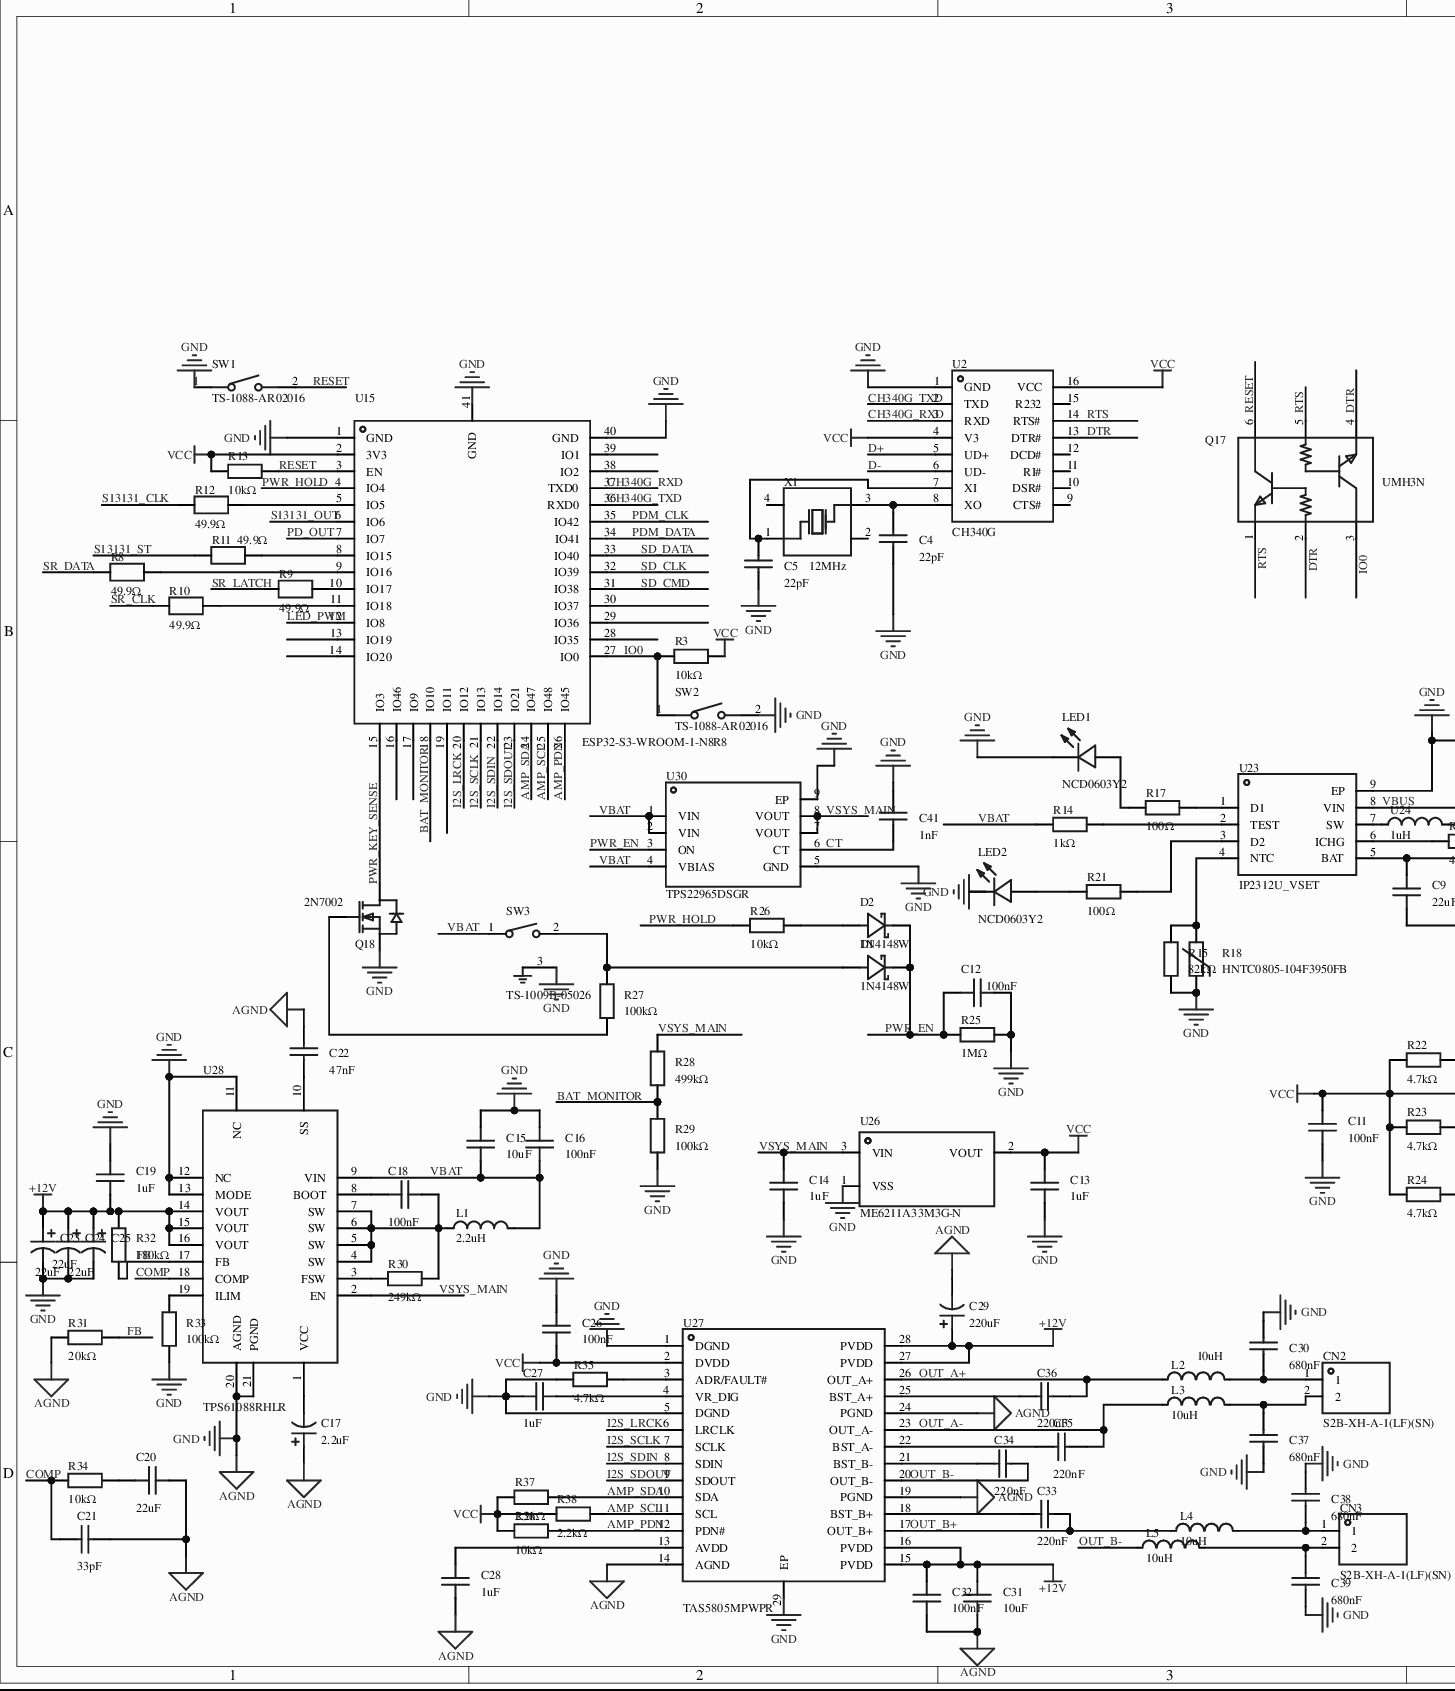
[diagram p0: MISC75432-3.schdoc, left]
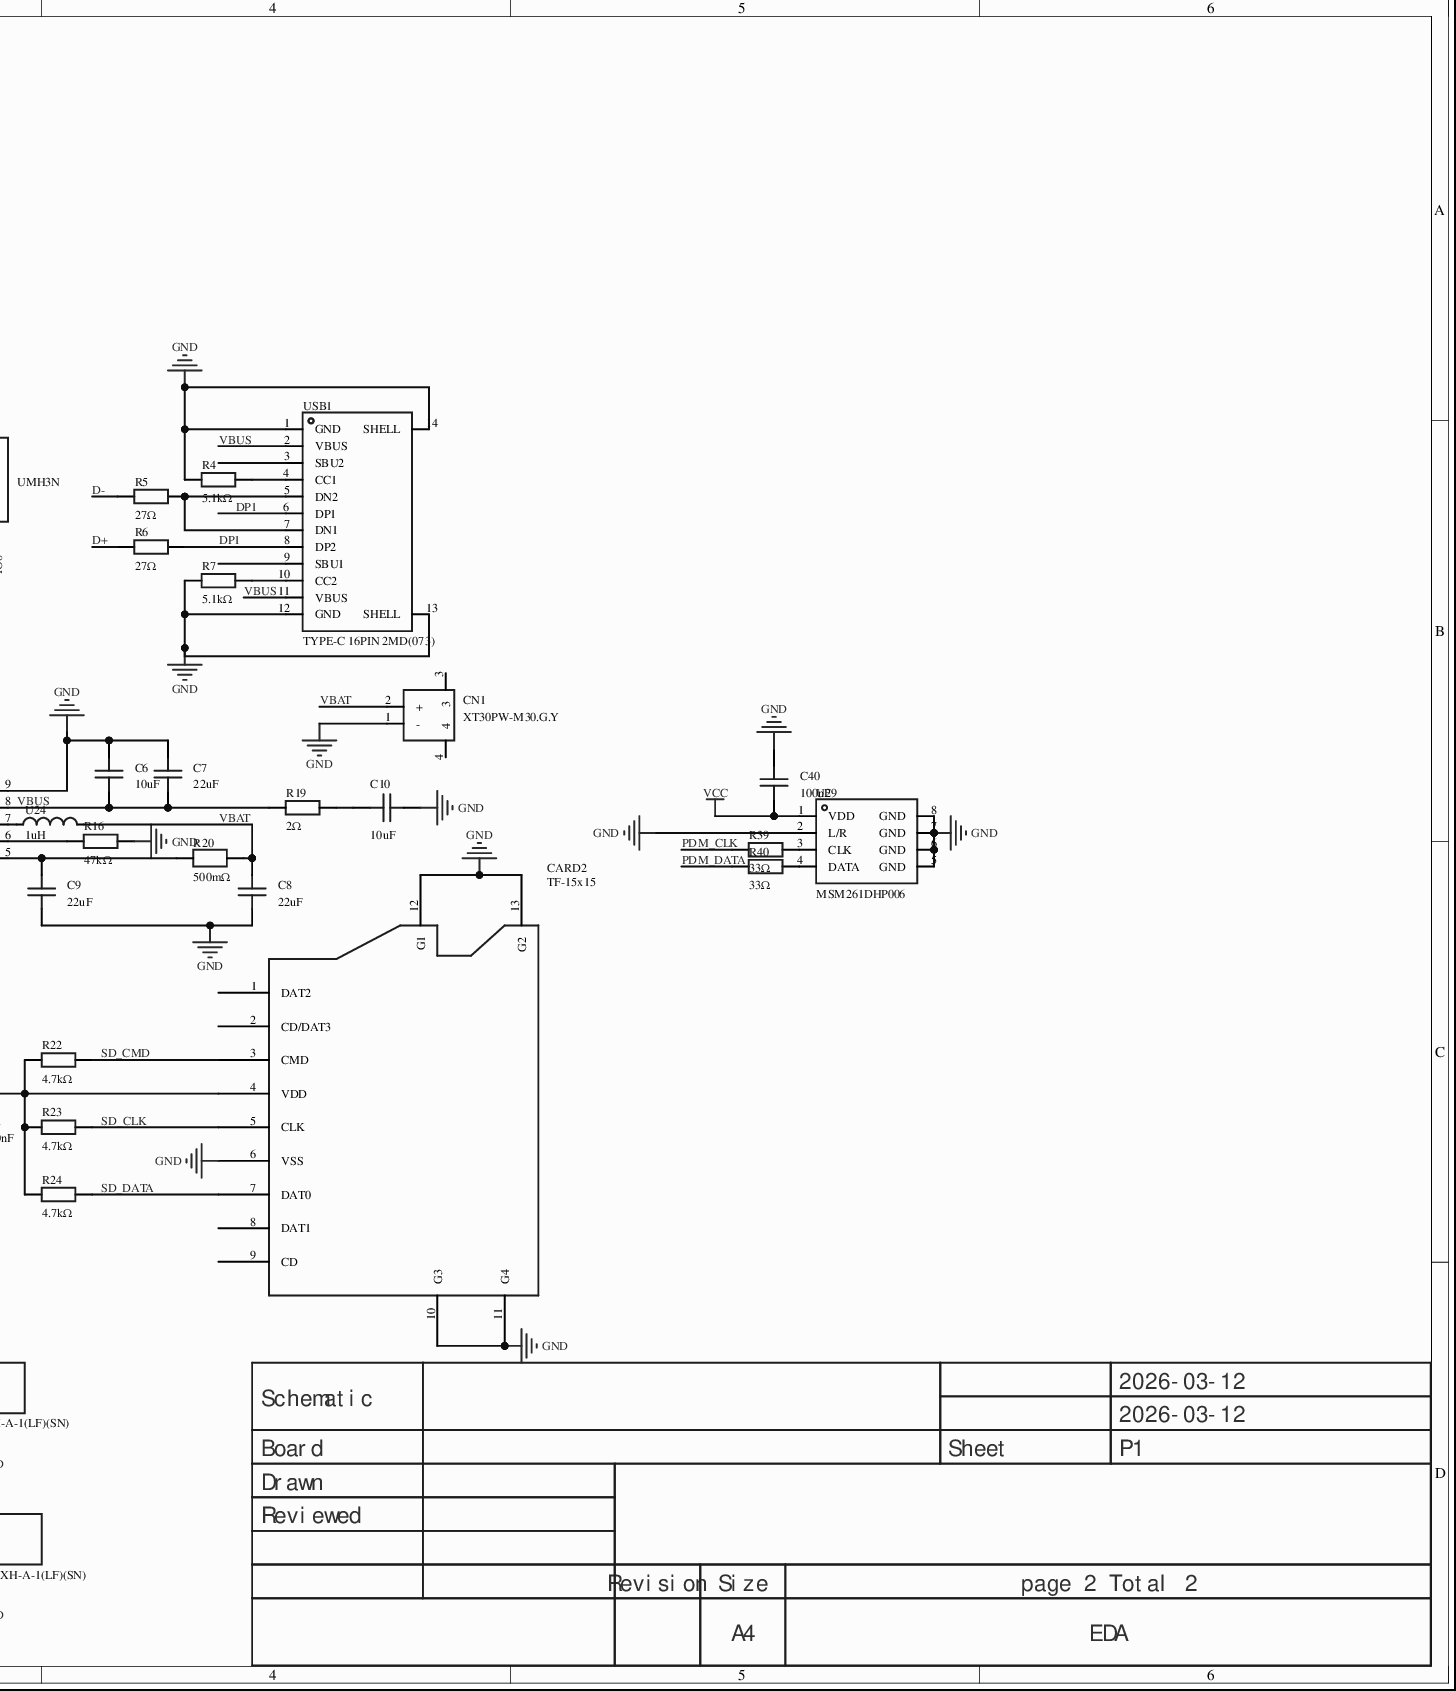
[diagram p1: MISC75432-3.schdoc, right]
# Altium project MISC75432-2.PrjPcb (part 1 of 3)
2 sheets, 150 parts. Net scope: global (net labels, ports and power ports of the same name join across sheets).
Board file: MISC75432.pcbdoc
Sheets:
  MISC75432-3.schdoc
  MISC75432-4.schdoc

## Sheet MISC75432-3.schdoc
size 424 x 254 mm; Version: V1.0; @Project Name: MISC75432; @Update Date: 2026-03-12; @Create Date: 2026-03-12; @Board Name: MISC75432; @Create Time: 13:14:40; @Page Count: 2; @Page No: 2; @Schematic Name: MISC75432; @Update Time: 13:14:40; Size: A4

### Parts
C4  22pF  [C0603]
C5  22pF  [C0603]
C6  10uF  [C0603]
C7  22uF  [C0603]
C8  22uF  [C0603]
C9  22uF  [C0603]
C10  10uF  [C0603]
C11  100nF  [C0603]
C12  100nF  [C0603]
C13  1uF  [C0603]
C14  1uF  [C0603]
C15  10uF  [C0603]
C16  100nF  [C0603]
C17  2.2uF  [CAP-SMD_BD5.0-L5.3-W5.3-LS6.0-FD]
C18  100nF  [C0603]
C19  1uF  [C0603]
C20  22uF  [C0603]
C21  33pF  [C0603]
C22  47nF  [C0603]
C23  22uF  [CAP-SMD_BD5.0-L5.3-W5.3-LS6.3-FD-1]
C24  22uF  [CAP-SMD_BD5.0-L5.3-W5.3-LS6.3-FD-1]
C25  22uF  [CAP-SMD_BD5.0-L5.3-W5.3-LS6.3-FD-1]
C26  100nF  [C0603]
C27  1uF  [C0603]
C28  1uF  [C0603]
C29  220uF  [CAP-SMD_BD6.3-L6.6-W6.6-LS7.3-FD-H7.7]
C30  680nF  [C0603]
C31  10uF  [C0603]
C32  100nF  [C0603]
C33  220nF  [C0603]
C34  220nF  [C0603]
C35  220nF  [C0603]
C36  220nF  [C0603]
C37  680nF  [C0603]
C38  680nF  [C0603]
C39  680nF  [C0603]
C40  100nF  [C0603]
C41  1nF  [C0603]
CARD2  TF-15x15  [TF-SMD_TF-15-15]
CN1  XT30PW-M30.G.Y  [CONN-TH_XT30PW-M]
CN2  S2B-XH-A-1(LF)(SN)  [CONN-TH_S2B-XH-A-1-LF-SN]
CN3  S2B-XH-A-1(LF)(SN)  [CONN-TH_S2B-XH-A-1-LF-SN]
D1  1N4148W  [SOD-123_L2.7-W1.6-LS3.7-FD]
D2  1N4148W  [SOD-123_L2.7-W1.6-LS3.7-FD]
L1  2.2uH  [IND-SMD_L4.6-W4.1_MHCI04015]
L2  10uH  [IND-SMD_L7.3-W6.8]
L3  10uH  [IND-SMD_L7.3-W6.8]
L4  10uH  [IND-SMD_L7.3-W6.8]
L5  10uH  [IND-SMD_L7.3-W6.8]
LED1  NCD0603Y2  [LED0603-RD]
LED2  NCD0603Y2  [LED0603-RD]
Q17  UMH3N  [SC-70-6_L2.2-W1.3-P0.65-LS2.1-BR]
Q18  2N7002  [SOT-23-3_L2.9-W1.3-P1.90-LS2.4-BR]
R3  10kΩ  [R0603]
R4  5.1kΩ  [R0603]
R5  27Ω  [R0603]
R6  27Ω  [R0603]
R7  5.1kΩ  [R0603]
R8  49.9Ω  [R0603]
R9  49.9Ω  [R0603]
R10  49.9Ω  [R0603]
R11  49.9Ω  [R0603]
R12  49.9Ω  [R0603]
R13  10kΩ  [R0603]
R14  1kΩ  [R0603]
R15  82kΩ  [R0603]
R16  47kΩ  [R0603]
R17  100Ω  [R0603]
R18  HNTC0805-104F3950FB  [R0805]
R19  2Ω  [R0603]
R20  500mΩ  [R1206]
R21  100Ω  [R0603]
R22  4.7kΩ  [R0603]
R23  4.7kΩ  [R0603]
R24  4.7kΩ  [R0603]
R25  1MΩ  [R0603]
R26  10kΩ  [R0603]
R27  100kΩ  [R0603]
R28  499kΩ  [R0603]
R29  100kΩ  [R0603]
R30  249kΩ  [R0603]
R31  20kΩ  [R0603]
R32  180kΩ  [R0603]
R33  100kΩ  [R0603]
R34  10kΩ  [R0603]
R35  4.7kΩ  [R0603]
R36  10kΩ  [R0603]
R37  2.2kΩ  [R0603]
R38  2.2kΩ  [R0603]
R39  33Ω  [R0603]
R40  33Ω  [R0603]
SW1  TS-1088-AR02016  [SW-SMD_L3.9-W3.0-P4.45]
SW2  TS-1088-AR02016  [SW-SMD_L3.9-W3.0-P4.45]
SW3  TS-1009B-05026  [SW-TH_3P-L4.5-W3.8-P3.10-LS1.9_TS-1009B-05026]
U2  CH340G  [SOIC-16_L9.9-W3.9-P1.27-LS6.0-BL]
U15  ESP32-S3-WROOM-1-N8R8  [WIRELM-SMD_ESP32-S3-WROOM-1]
U23  IP2312U_VSET  [SOP-8_L4.9-W3.9-P1.27-LS6.0-BL-EP]
U24  1uH  [IND-SMD_L2.5-W2.0-VLS252012CX-150M]
U26  ME6211A33M3G-N  [SOT-23-3_L2.9-W1.6-P1.90-LS2.8-BR]
U27  TAS5805MPWPR  [HTSSOP-28_L9.7-W4.4-P0.65-LS6.4-BL-EP]
U28  TPS61088RHLR  [VQFN-20_L4.6-W3.6-P0.50-BL]
U29  MSM261DHP006  [QFN-8_L4.0-W3.0_WMM7040DTHN0-8-TR]
U30  TPS22965DSGR  [UDFN-8_L2.0-W2.0-P0.50-TL-EP]
USB1  TYPE-C 16PIN 2MD(073)  [USB-C-SMD_TYPE-C-6PIN-2MD-073]
X1  12MHz  [CRYSTAL-SMD_4P-L3.2-W2.5-BL]

### Nets
+12V: C19.1 C23.1 C24.1 C25.1 C29.1 C31.2 C32.2 R32.2 U27.15(PVDD) U27.16(PVDD) U27.27(PVDD) U27.28(PVDD) U28.14(VOUT) U28.15(VOUT) U28.16(VOUT)
GND: C4.1 C5.1 C6.2 C7.2 C8.1 C9.1 C10.2 C11.1 C12.2 C13.1 C14.1 C15.2 C16.2 C17.1 C19.2 C20.2 C21.2 C22.2 C23.2 C24.2 C25.2 C26.2 C27.2 C28.1 C29.2 C30.2 C31.1 C32.1 C37.1 C38.2 C39.1 C40.2 C41.2 CARD2.6(VSS) CARD2.10(G3) CARD2.11(G4) CARD2.12(G1) CARD2.13(G2) CN1.1(-) LED1.1(K) LED2.1(K) Q18.2(S) R4.1 R7.1 R15.1 R16.2 R18.1 R25.2 R29.1 R31.1 R33.1 R35.1 SW1.1 SW2.2 SW3.3 U2.1(GND) U15.1(GND) U15.40(GND) U15.41(GND) U23.9(EP) U26.1(VSS) U27.1(DGND) U27.5(DGND) U27.14(AGND) U27.19(PGND) U27.24(PGND) U27.29(EP) U28.11(NC) U28.12(NC) U28.13(MODE) U28.20(AGND) U28.21(PGND) U29.2(L/R) U29.5(GND) U29.6(GND) U29.7(GND) U29.8(GND) U30.5(GND) U30.9(EP) USB1.1(GND) USB1.12(GND) USB1.13(SHELL) USB1.14(SHELL)  [also labelled AGND]
VCC: C11.2 C13.2 C26.1 C40.1 CARD2.4(VDD) R3.2 R13.1 R22.1 R23.1 R24.1 R36.1 R37.1 R38.1 U2.4(V3) U2.16(VCC) U15.2(3V3) U26.2(VOUT) U27.2(DVDD) U29.1(VDD)
AMP_PDN: R36.2 U15.26(IO45) U27.12(PDN#)
AMP_SCL: R38.2 U15.25(IO48) U27.11(SCL)
AMP_SDA: R37.2 U15.24(IO47) U27.10(SDA)
BAT_MONITOR: R28.1 R29.2 U15.18(IO10)
CH340G_RXD: U2.3(RXD) U15.37(TXD0)
CH340G_TXD: U2.2(TXD) U15.36(RXD0)
COMP: C21.1 R34.1 U28.18(COMP)
CT: C41.1 U30.6(CT)
D+: R6.1 U2.5(UD+)
D-: R5.1 U2.6(UD-)
DP1: R6.2 USB1.6(DP1) USB1.8(DP2)
DTR: Q17.2(B) Q17.4(E) U2.13(DTR#)
FB: R31.2 R32.1 U28.17(FB)
I2S_LRCK: U15.20(IO12) U27.6(LRCLK)
I2S_SCLK: U15.21(IO13) U27.7(SCLK)
I2S_SDIN: U15.22(IO14) U27.8(SDIN)
I2S_SDOUT: U15.23(IO21) U27.9(SDOUT)
IO0: Q17.3(C) R3.1 SW2.1 U15.27(IO0)
LED_PWM: U15.12(IO8)
OUT_A+: C36.2 L2.1 U27.26(OUT_A+)
OUT_A-: C35.2 L3.1 U27.23(OUT_A-)
OUT_B+: C33.2 L4.1 U27.17(OUT_B+)
OUT_B-: C34.2 L5.1 U27.20(OUT_B-)
PD_OUT: U15.7(IO7)
PDM_CLK: R39.1 U15.35(IO42)
PDM_DATA: R40.1 U15.34(IO41)
PWR_EN: C12.1 D1.2(K) D2.2(K) R25.1 U30.3(ON)
PWR_HOLD: R26.1 U15.4(IO4)
PWR_KEY_SENSE: Q18.3(D) U15.15(IO3)
RESET: Q17.6(C) R13.2 SW1.2 U15.3(EN)
RTS: Q17.1(E) Q17.5(B) U2.14(RTS#)
S13131_CLK: R12.1
S13131_OUT: U15.6(IO6)
S13131_ST: R11.1
SD_CLK: CARD2.5(CLK) R23.2 U15.32(IO39)
SD_CMD: CARD2.3(CMD) R22.2 U15.31(IO38)
SD_DATA: CARD2.7(DAT0) R24.2 U15.33(IO40)
SR_CLK: R10.1
SR_DATA: R8.2
SR_LATCH: R9.2
VBAT: C8.2 C15.1 C16.1 CN1.2(+) L1.2 R14.1 R20.2 SW3.1 U24.2 U28.9(VIN) U30.1(VIN) U30.2(VIN) U30.4(VBIAS)
VBUS: C6.1 C7.1 R19.1 U23.8(VIN) USB1.2(VBUS) USB1.11(VBUS)
VSYS_MAIN: C14.2 R28.2 U26.3(VIN) U28.2(EN) U30.7(VOUT) U30.8(VOUT)
NetC4_2: C4.2 U2.8(XO) X1.3(OSC2)
NetC5_2: C5.2 U2.7(XI) X1.1(OSC1)
NetC9_2: C9.2 R20.1 U23.5(BAT)
NetC10_1: C10.1 R19.2
NetC17_2: C17.2 U28.1(VCC)
NetC18_1: C18.1 U28.8(BOOT)
NetC18_2: C18.2 L1.1 R30.2 U28.4(SW) U28.5(SW) U28.6(SW) U28.7(SW)
NetC20_1: C20.1 R34.2
NetC22_1: C22.1 U28.10(SS)
NetC27_1: C27.1 U27.4(VR_DIG)
NetC28_2: C28.2 U27.13(AVDD)
NetC30_1: C30.1 CN2.1 L2.2
NetC33_1: C33.1 U27.18(BST_B+)
NetC34_1: C34.1 U27.21(BST_B-)
NetC35_1: C35.1 U27.22(BST_A-)
NetC36_1: C36.1 U27.25(BST_A+)
NetC37_2: C37.2 CN2.2 L3.2
NetC38_1: C38.1 CN3.1 L4.2
NetC39_2: C39.2 CN3.2 L5.2
NetD1_1: D1.1(A) R27.2 SW3.2
NetD2_1: D2.1(A) R26.2
NetLED1_2: LED1.2(A) R17.1
NetLED2_2: LED2.2(A) R21.1
NetQ18_1: Q18.1(G) R27.1
NetR4_2: R4.2 USB1.4(CC1)
NetR5_2: R5.2 USB1.5(DN2) USB1.7(DN1)
NetR7_2: R7.2 USB1.10(CC2)
NetR8_1: R8.1 U15.9(IO16)
NetR9_1: R9.1 U15.10(IO17)
NetR10_2: R10.2 U15.11(IO18)
NetR11_2: R11.2 U15.8(IO15)
NetR12_2: R12.2 U15.5(IO5)
NetR14_2: R14.2 U23.2(TEST)
NetR15_2: R15.2 R18.2 U23.4(NTC)
NetR16_1: R16.1 U23.6(ICHG)
NetR17_2: R17.2 U23.1(D1)
NetR21_2: R21.2 U23.3(D2)
NetR30_1: R30.1 U28.3(FSW)
NetR33_2: R33.2 U28.19(ILIM)
NetR35_2: R35.2 U27.3(ADR/FAULT#)
NetR39_2: R39.2 U29.3(CLK)
NetR40_2: R40.2 U29.4(DATA)
NetU23_7: U23.7(SW) U24.1

Not connected (* = marked no-connect by the designer): CARD2 1(DAT2) 2(CD/DAT3) 8(DAT1) 9(CD); CN1 3 4; U2 9(CTS#) 10(DSR#) 11(RI#) 12(DCD#) 15(R232); U15 13(IO19) 14(IO20) 16(IO46) 17(IO9) 19(IO11) 28(IO35) 29(IO36) 30(IO37) 38(IO2) 39(IO1); USB1 3(SBU2) 9(SBU1); X1 2(GND) 4(GND)

### Notes on the sheet
- 2026-03-12
- Schematic
- Board
- Sheet
- P1
- Drawn
- Reviewed
- Revision
- Size
- A4
- page 2 Total 2
- EDA